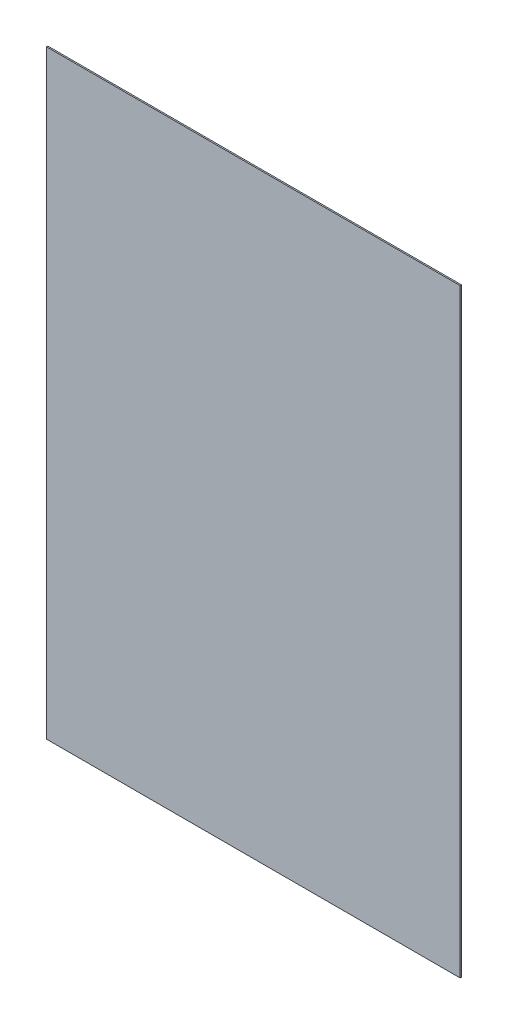
from build123d import *

# Parameters (mm, degrees)
SKETCH_1_W      = 935
SKETCH_1_H      = 1355
EXTRUDE_1_DEPTH = 3


with BuildPart() as part:
    # 草图1 → 凸台-拉伸1 (new body)
    with BuildSketch(Plane.XY):
        Rectangle(SKETCH_1_W, SKETCH_1_H)
    extrude(amount=EXTRUDE_1_DEPTH)


solid = part.part
